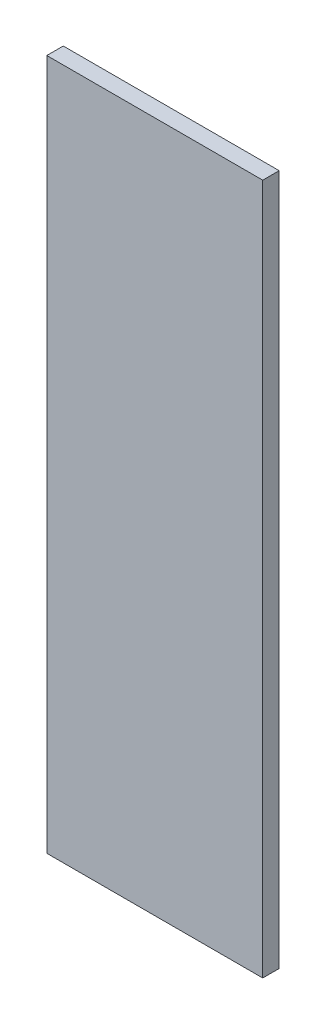
SolidWorks part; units mm, degrees
material "Q235"
ref_plane "Front Plane" through (0, 0, 0) normal (0, 0, 1) x (1, 0, 0)
ref_plane "Top Plane" through (0, 0, 0) normal (0, 1, 0) x (1, 0, 0)
ref_plane "Right Plane" through (0, 0, 0) normal (1, 0, 0) x (0, 0, -1)
sketch "Sketch1" plane through (0, 0, 0) normal (0, 0, 1) x (1, 0, 0)
  line L1 (-52.5, 168) -> (52.5, 168)
  line L2 (-52.5, 168) -> (-52.5, -168)
  line L3 (-52.5, -168) -> (52.5, -168)
  line L4 (52.5, 168) -> (52.5, -168)
  dimension "D1" = 336
  dimension "D2" = 168
  dimension "D3" = 105
  dimension "D4" = 52.5
extrude "Boss-Extrude1" add sketch "Sketch1" along normal mid plane 8
